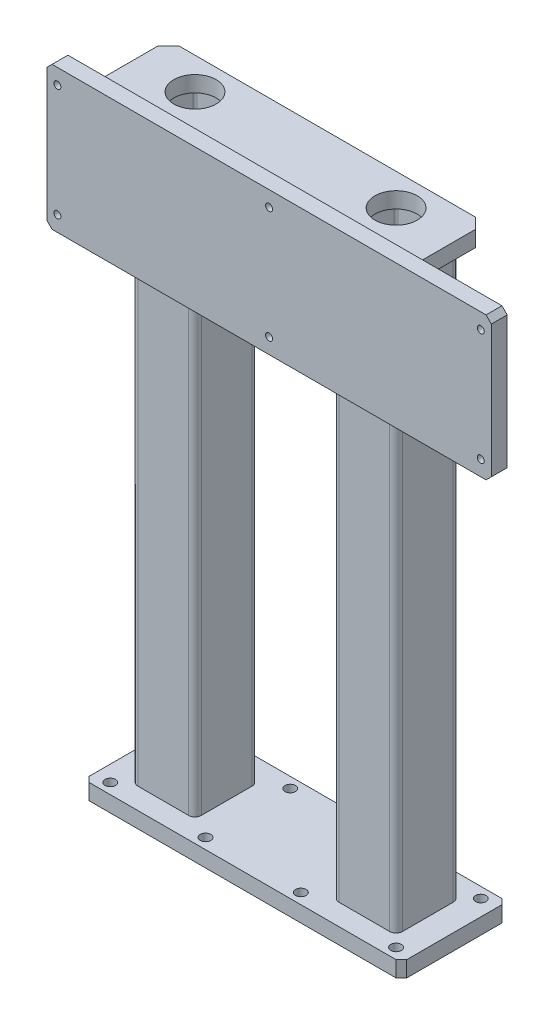
SolidWorks part; units mm, degrees
material "Q235A+方通"
ref_plane "前视基准面" through (0, 0, 0) normal (0, 0, 1) x (1, 0, 0)
ref_plane "上视基准面" through (0, 0, 0) normal (0, 1, 0) x (1, 0, 0)
ref_plane "右视基准面" through (0, 0, 0) normal (1, 0, 0) x (0, 0, -1)
sketch "草图1" plane through (0, 0, 0) normal (0, 1, 0) x (1, 0, 0)
  line L1 (-150, 50) -> (150, 50)
  line L2 (-150, 50) -> (-150, -50)
  line L3 (-150, -50) -> (150, -50)
  line L4 (150, 50) -> (150, -50)
  line L5 (-150, 50) -> (150, -50) construction
  line L6 (-150, -50) -> (150, 50) construction
  point P0 (0, 0)
  dimension "D1" = 300
  dimension "D2" = 100
extrude "凸台-拉伸1" add sketch "草图1" along normal blind 15
sketch "草图2" plane through (0, 15, 0) normal (0, 1, 0) x (1, 0, 0)
  line L0 (-150, -50) -> (150, -50) construction
  line L1 (-119, 30) -> (-71, 30)
  line L2 (-125, 24) -> (-125, -24)
  line L3 (-119, -30) -> (-71, -30)
  line L4 (-65, 24) -> (-65, -24)
  line L5 (-150, 50) -> (-150, -50) construction
  line L6 (-119, 26) -> (-71, 26)
  line L7 (-69, 24) -> (-69, -24)
  line L8 (-119, -26) -> (-71, -26)
  line L9 (-121, 24) -> (-121, -24)
  line L10 (0, 50) -> (0, -50) construction
  line L11 (150, 50) -> (-150, 50) construction
  line L12 (121, 24) -> (121, -24)
  line L13 (119, -26) -> (71, -26)
  line L14 (69, 24) -> (69, -24)
  line L15 (119, 26) -> (71, 26)
  line L16 (65, 24) -> (65, -24)
  line L17 (119, -30) -> (71, -30)
  line L18 (125, 24) -> (125, -24)
  line L19 (119, 30) -> (71, 30)
  arc A0 (-71, 30) -> (-65, 24) centre (-71, 24) cw
  arc A1 (-125, -24) -> (-119, -30) centre (-119, -24) ccw
  arc A2 (-71, -30) -> (-65, -24) centre (-71, -24) ccw
  arc A3 (-119, 30) -> (-125, 24) centre (-119, 24) ccw
  arc A4 (-71, 26) -> (-69, 24) centre (-71, 24) cw
  arc A5 (-71, -26) -> (-69, -24) centre (-71, -24) ccw
  arc A6 (-121, -24) -> (-119, -26) centre (-119, -24) ccw
  arc A7 (-119, 26) -> (-121, 24) centre (-119, 24) ccw
  arc A8 (119, 26) -> (121, 24) centre (119, 24) cw
  arc A9 (121, -24) -> (119, -26) centre (119, -24) cw
  arc A10 (71, -26) -> (69, -24) centre (71, -24) cw
  arc A11 (71, 26) -> (69, 24) centre (71, 24) ccw
  arc A12 (119, 30) -> (125, 24) centre (119, 24) cw
  arc A13 (71, -30) -> (65, -24) centre (71, -24) cw
  arc A14 (125, -24) -> (119, -30) centre (119, -24) cw
  arc A15 (71, 30) -> (65, 24) centre (71, 24) ccw
  point P12 (-125, -30)
  point P15 (-65, -30)
  point P47 (65, -30)
  point P56 (125, -30)
  dimension "D4" = 6
  dimension "D1" = 60
  dimension "D2" = 20
  dimension "D3" = 25
  dimension "D5" = 60
  dimension "D6" = 4
extrude "凸台-拉伸2" add sketch "草图2" along normal blind 550
sketch "草图3" plane through (0, 565, 0) normal (0, 1, 0) x (1, 0, 0)
  line L0 (-125, 24) -> (-125, -24) construction
  line L1 (-150, -70) -> (150, -70)
  line L2 (-150, -70) -> (-150, 30)
  line L3 (-150, 30) -> (150, 30)
  line L4 (150, -70) -> (150, 30)
  line L5 (-95, 0) -> (95, 0) construction
  line L6 (-71, 30) -> (-119, 30) construction
  line L7 (95, 0) -> (95, 26) construction
  line L8 (119, 26) -> (71, 26) construction
  line L9 (-95, 0) -> (-95, 26) construction
  line L10 (-71, 26) -> (-119, 26) construction
  circle A0 centre (-95, 0) radius 20
  circle A1 centre (95, 0) radius 20
  dimension "D5" = 40
  dimension "D1" = 25
  dimension "D2" = 300
  dimension "D3" = 100
  dimension "D4" = 30
extrude "凸台-拉伸3" add sketch "草图3" along normal blind 15
sketch "草图4" plane through (0, 0, 70) normal (0, 0, 1) x (1, 0, 0)
  line L0 (-150, 580) -> (150, 580) construction
  line L1 (-150, 485) -> (270, 485)
  line L2 (-150, 485) -> (-150, 620)
  line L3 (-150, 620) -> (270, 620)
  line L4 (270, 485) -> (270, 620)
  line L6 (-150, 580) -> (-150, 565) construction
  dimension "D1" = 135
  dimension "D2" = 40
  dimension "D3" = 420
extrude "凸台-拉伸4" add sketch "草图4" along normal blind 15
hole_wizard "打孔尺寸(%根据)内六角圆柱头螺钉的类型1" positions "草图6" profile "草图5" counterbore size "M6" standard "GB"
sketch "草图6" plane through (0, 0, 70) normal (0, 0, -1) x (-1, 0, 0)
  line L0 (-270, 620) -> (150, 620) construction
  line L1 (150, 620) -> (150, 580) construction
  line L2 (140, 605.5) -> (140, 499.5) construction
  point P0 (140, 605.5)
  point P7 (140, 499.5)
  dimension "D1" = 14.5
  dimension "D2" = 10
  dimension "D3" = 106
sketch "草图5" plane through (-140, 605.5, 70) normal (1, 0, 0) x (0, 1, 0)
  line L0 (0, 0) -> (0, 16.9828)
  line L1 (0, 16.9828) -> (3.3, 15)
  line L2 (3.3, 15) -> (3.3, 6.8)
  line L3 (3.3, 6.8) -> (5.5, 6.8)
  line L4 (5.5, 6.8) -> (5.5, 0)
  line L5 (5.5, 0) -> (0, 0)
  line L10 (0, 16.9828) -> (-3.3, 15) construction
  line L11 (0, -6.35) -> (0, 107.95) construction
  dimension "孔直径" = 6.6
  dimension "孔深度" = 15
  dimension "柱形沉头孔直径" = 11
  dimension "柱形沉头孔深度" = 6.8
  dimension "导头角度" = 118
pattern_linear "阵列(线性)1" count 3 spacing 200 along (1, 0, 0) of "打孔尺寸(%根据)内六角圆柱头螺钉的类型1"
sketch "草图7" plane through (0, 15, 0) normal (0, 1, 0) x (1, 0, 0)
  circle A1 centre (-95, 0) radius 20
  circle A2 centre (-95, 0) radius 20
  circle A3 centre (95, 0) radius 20
  circle A4 centre (95, 0) radius 20
  dimension "D1" = 0
  dimension "D2" = 0
extrude "切除-拉伸1" cut sketch "草图7" against normal through all
chamfer "倒角1" distance 10 angle 45 2 edges at (-150, 572.5, -30) (150, 572.5, -30)
chamfer "倒角2" distance 5 angle 45 4 edges at (270, 485, 77.5) (270, 620, 77.5) (-150, 485, 77.5) (-150, 620, 77.5)
sketch "草图8" plane through (0, 0, 70) normal (0, 0, -1) x (-1, 0, 0)
  line L0 (71, 565) -> (119, 565) construction
  line L1 (-102.5, 565) -> (-87.5, 565)
  line L2 (-102.5, 565) -> (-102.5, 485)
  line L3 (-102.5, 485) -> (-87.5, 485)
  line L4 (-87.5, 565) -> (-87.5, 485)
  line L5 (87.5, 565) -> (102.5, 565)
  line L6 (87.5, 565) -> (87.5, 485)
  line L7 (87.5, 485) -> (102.5, 485)
  line L8 (102.5, 565) -> (102.5, 485)
  line L9 (145, 485) -> (-265, 485) construction
  line L12 (-119, 565) -> (-71, 565) construction
  line L13 (-95, 485) -> (-95, 15) construction
  line L14 (-119, 15) -> (-71, 15) construction
  line L15 (95, 485) -> (95, 15) construction
  line L16 (71, 15) -> (119, 15) construction
  dimension "D1" = 15
extrude "凸台-拉伸5" add sketch "草图8" along normal up to next
sketch "草图9" plane through (0, 15, 0) normal (0, 1, 0) x (1, 0, 0)
  line L0 (150, 50) -> (-150, 50) construction
  line L1 (-150, 50) -> (-150, -50) construction
  circle A0 centre (-135, 40) radius 5
  dimension "D1" = 10
  dimension "D2" = 10
  dimension "D3" = 15
extrude "切除-拉伸2" cut sketch "草图9" against normal through all
pattern_linear "阵列(线性)2" count 4 spacing 90 along (1, 0, 0) count 2 spacing 80 along (0, 0, 1) of "切除-拉伸2"
chamfer "倒角3" distance 5 angle 45 4 edges at (150, 7.5, 50) (150, 7.5, -50) (-150, 7.5, 50) (-150, 7.5, -50)
sketch "草图10" plane through (0, 0, -30) normal (0, 0, -1) x (-1, 0, 0)
  line L0 (-95, 50) -> (-95, 15) construction
  line L1 (-107.5, 50) -> (-82.5, 50)
  line L2 (-112.5, 55) -> (-112.5, 95)
  line L3 (-107.5, 100) -> (-82.5, 100)
  line L4 (-77.5, 55) -> (-77.5, 95)
  line L5 (-112.5, 50) -> (-77.5, 100) construction
  line L6 (-112.5, 100) -> (-77.5, 50) construction
  line L7 (82.5, 50) -> (107.5, 50)
  line L8 (77.5, 55) -> (77.5, 95)
  line L9 (82.5, 100) -> (107.5, 100)
  line L10 (112.5, 55) -> (112.5, 95)
  line L11 (77.5, 50) -> (112.5, 100) construction
  line L12 (77.5, 100) -> (112.5, 50) construction
  line L13 (-119, 15) -> (-71, 15) construction
  line L14 (95, 50) -> (95, 15) construction
  line L15 (71, 15) -> (119, 15) construction
  arc A0 (107.5, 50) -> (112.5, 55) centre (107.5, 55) ccw
  arc A1 (77.5, 95) -> (82.5, 100) centre (82.5, 95) cw
  arc A2 (82.5, 50) -> (77.5, 55) centre (82.5, 55) cw
  arc A3 (107.5, 100) -> (112.5, 95) centre (107.5, 95) cw
  arc A4 (-82.5, 50) -> (-77.5, 55) centre (-82.5, 55) ccw
  arc A5 (-112.5, 95) -> (-107.5, 100) centre (-107.5, 95) cw
  arc A6 (-107.5, 50) -> (-112.5, 55) centre (-107.5, 55) cw
  arc A7 (-82.5, 100) -> (-77.5, 95) centre (-82.5, 95) cw
  point P0 (-95, 75)
  point P5 (95, 75)
  dimension "D4" = 5
  dimension "D1" = 35
  dimension "D2" = 35
  dimension "D3" = 50
extrude "切除-拉伸3" cut sketch "草图10" against normal blind 5
